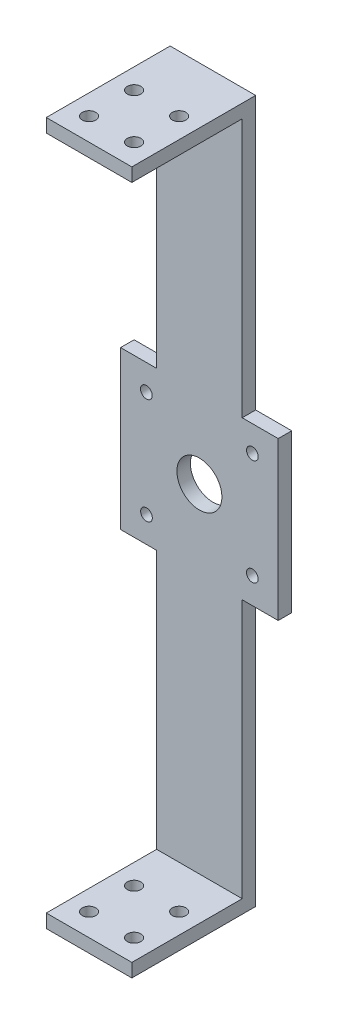
SolidWorks part; units mm, degrees
ref_plane "前视基准面" through (0, 0, 0) normal (0, 0, 1) x (1, 0, 0)
ref_plane "上视基准面" through (0, 0, 0) normal (0, 1, 0) x (1, 0, 0)
ref_plane "右视基准面" through (0, 0, 0) normal (1, 0, 0) x (0, 0, -1)
sketch "草图1" plane through (0, 0, 0) normal (0, 1, 0) x (1, 0, 0)
  line L1 (-19, 27.5) -> (19, 27.5)
  line L2 (-19, 27.5) -> (-19, -27.5)
  line L3 (-19, -27.5) -> (19, -27.5)
  line L4 (19, 27.5) -> (19, -27.5)
  line L5 (-19, 27.5) -> (19, -27.5) construction
  line L6 (-19, -27.5) -> (19, 27.5) construction
  point P0 (0, 0)
  dimension "D1" = 55
  dimension "D2" = 38
extrude "凸台-拉伸1" add sketch "草图1" along normal blind 6
sketch "草图2" plane through (0, 6, 0) normal (0, 1, 0) x (1, 0, 0)
  line L0 (0, 27.5) -> (0, -27.5) construction
  line L1 (19, 27.5) -> (-19, 27.5) construction
  line L2 (-19, -27.5) -> (19, -27.5) construction
  circle A0 centre (-10, 2.5) radius 3
  circle A1 centre (10, 2.5) radius 3
  circle A2 centre (10, -17.5) radius 3
  circle A3 centre (-10, -17.5) radius 3
  dimension "D1" = 6
  dimension "D2" = 6
  dimension "D3" = 6
  dimension "D4" = 20
  dimension "D5" = 20
  dimension "D6" = 10
  dimension "D7" = 20
extrude "切除-拉伸1" cut sketch "草图2" against normal blind 16
sketch "草图3" plane through (0, 6, 0) normal (0, 1, 0) x (1, 0, 0)
  line L0 (19, -27.5) -> (19, 27.5) construction
  line L1 (-19, 27.5) -> (19, 27.5)
  line L2 (-19, 27.5) -> (-19, 21.5)
  line L3 (-19, 21.5) -> (19, 21.5)
  line L4 (19, 27.5) -> (19, 21.5)
  dimension "D1" = 6
extrude "凸台-拉伸2" add sketch "草图3" along normal blind 300
sketch "草图5" plane through (0, 306, 0) normal (0, 1, 0) x (1, 0, 0)
  line L4 (-19, 27.5) -> (-19, 21.5)
  line L5 (-19, 21.5) -> (19, 21.5)
  line L6 (19, 21.5) -> (19, 27.5)
  line L7 (19, 27.5) -> (-19, 27.5)
  line L8 (-19, 27.5) -> (-19, 21.5)
  line L10 (19, 21.5) -> (19, 27.5)
  line L11 (19, 27.5) -> (-19, 27.5)
  line L12 (19, 21.5) -> (-19, 21.5)
  line L13 (-19, 21.5) -> (-19, -27.5)
  line L14 (-19, -27.5) -> (19, -27.5)
  line L15 (19, -27.5) -> (19, 21.5)
  line L17 (-19, 21.5) -> (-19, -27.5)
  line L18 (-19, -27.5) -> (19, -27.5)
  line L19 (19, -27.5) -> (19, 21.5)
  circle A0 centre (-10, 2.5) radius 3 construction
  circle A1 centre (-10, 2.5) radius 3
  circle A2 centre (10, 2.5) radius 3 construction
  circle A3 centre (10, 2.5) radius 3
  circle A4 centre (-10, -17.5) radius 3 construction
  circle A5 centre (-10, -17.5) radius 3
  circle A6 centre (10, -17.5) radius 3 construction
  circle A7 centre (10, -17.5) radius 3
  dimension "D1" = 0
  dimension "D2" = 0
extrude "凸台-拉伸3" add sketch "草图5" along normal blind 6
sketch "草图6" plane through (0, 0, -27.5) normal (0, 0, -1) x (-1, 0, 0)
  line L1 (-35, 121) -> (35, 121)
  line L2 (-35, 121) -> (-35, 191)
  line L3 (-35, 191) -> (35, 191)
  line L4 (35, 121) -> (35, 191)
  line L5 (-35, 121) -> (35, 191) construction
  line L6 (-35, 191) -> (35, 121) construction
  point P0 (0, 156)
  dimension "D1" = 70
  dimension "D2" = 70
extrude "凸台-拉伸4" add sketch "草图6" against normal up to surface (6 mm away) up to face at (0, 156, -21.5)
sketch "草图7" plane through (0, 0, -27.5) normal (0, 0, -1) x (-1, 0, 0)
  circle A0 centre (23.545, 179.545) radius 2.6
  circle A1 centre (23.5, 132.5) radius 2.6
  circle A2 centre (-23.5, 132.5) radius 2.6
  circle A3 centre (-23.545, 179.545) radius 2.6
  circle A4 centre (0, 156) radius 10
  dimension "D1" = 20
extrude "切除-拉伸2" cut sketch "草图7" against normal blind 10
